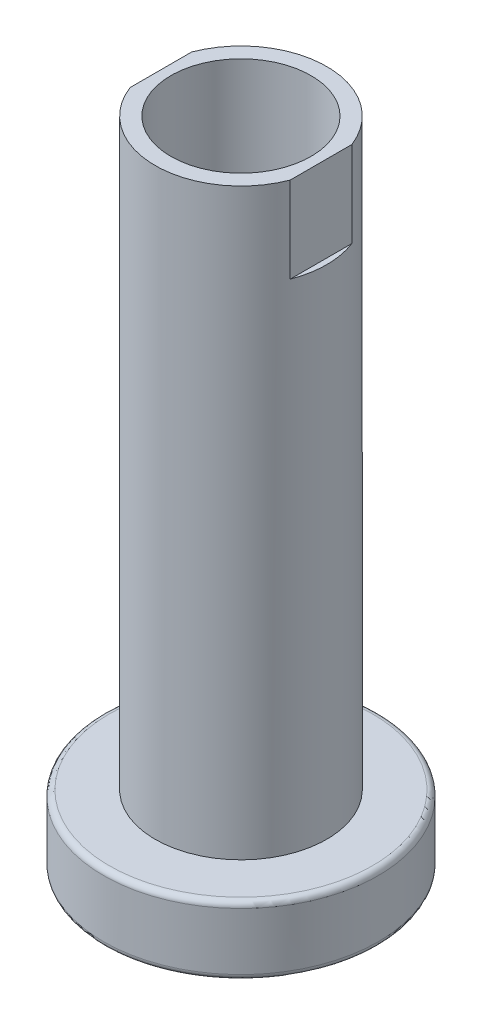
from build123d import *

# Parameters (mm, degrees)
CUT_EXTRUDE1_DEPTH      = 99.11063461
CUT_EXTRUDE1_DEPTH_BACK = 99.11063461
SKETCH2_W               = 1
SKETCH2_H               = 15
FILLET1_R               = 1
M27_TAPPED_HOLE1_D      = 24.5
M27_TAPPED_HOLE1_DEPTH  = 36
M27_TAPPED_HOLE1_TIP    = 7.360542583
M10_TAPPED_HOLE1_D      = 8.5
M10_TAPPED_HOLE1_DEPTH  = 20
M10_TAPPED_HOLE1_TIP    = 2.553657631


with BuildPart() as part:
    # Sketch1 → Revolve1 (revolve)
    with BuildSketch(Plane.XY):
        Polygon((0, 92.052683956), (0, -21.947316044), (-24, -21.947316044), (-24, -9.947316044), (-15, -9.947316044), (-15, 92.052683956), align=None)
    revolve(axis=Axis((0, 92.052683956, 0), (0, -1, 0)))

    # Sketch2 → Cut-Extrude1 (cut, two sides: drawn at the far end of the back side and taken through both)
    with BuildSketch(Plane.XY.offset(-CUT_EXTRUDE1_DEPTH_BACK)):
        with Locations((14.5, 84.552683956)):
            Rectangle(SKETCH2_W, SKETCH2_H)
        with Locations((-14.5, 84.552683956)):
            Rectangle(SKETCH2_W, SKETCH2_H)
    extrude(amount=CUT_EXTRUDE1_DEPTH + CUT_EXTRUDE1_DEPTH_BACK, mode=Mode.SUBTRACT)

    # Fillet1
    fillet1_edges = [part.edges().sort_by_distance(p)[0] for p in [
        (24, -9.947316044, 0),
        (24, -21.947316044, 0),
    ]]
    fillet(fillet1_edges, radius=FILLET1_R)

    # M27 Tapped Hole1
    with Locations(Plane(origin=(0, 92.052683956, 0), x_dir=(1, 0, 0), z_dir=(0, 1, 0))):
        with Locations((0, 0)):
            Hole(M27_TAPPED_HOLE1_D / 2, depth=M27_TAPPED_HOLE1_DEPTH)
            with Locations((0, 0, -(M27_TAPPED_HOLE1_DEPTH + M27_TAPPED_HOLE1_TIP / 2))):  # 118° drill point
                Cone(0, M27_TAPPED_HOLE1_D / 2, M27_TAPPED_HOLE1_TIP, mode=Mode.SUBTRACT)

    # M10 Tapped Hole1
    with Locations(Plane(origin=(0, -21.947316044, 0), x_dir=(-1, 0, 0), z_dir=(0, -1, 0))):
        with Locations((0, 0)):
            Hole(M10_TAPPED_HOLE1_D / 2, depth=M10_TAPPED_HOLE1_DEPTH)
            with Locations((0, 0, -(M10_TAPPED_HOLE1_DEPTH + M10_TAPPED_HOLE1_TIP / 2))):  # 118° drill point
                Cone(0, M10_TAPPED_HOLE1_D / 2, M10_TAPPED_HOLE1_TIP, mode=Mode.SUBTRACT)


solid = part.part
